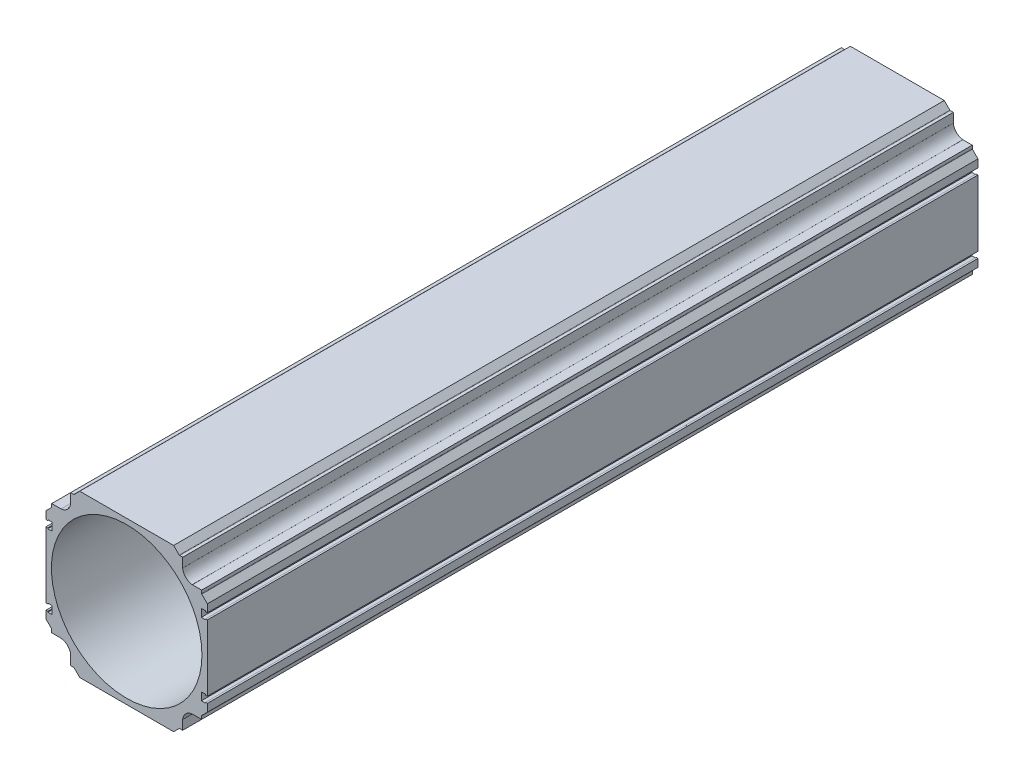
SolidWorks part; units mm, degrees
ref_plane "Front Plane" through (0, 0, 0) normal (0, 0, 1) x (1, 0, 0)
ref_plane "Top Plane" through (0, 0, 0) normal (0, 1, 0) x (1, 0, 0)
ref_plane "Right Plane" through (0, 0, 0) normal (1, 0, 0) x (0, 0, -1)
sketch "Sketch1" plane through (0, 0, 0) normal (0, 0, 1) x (1, 0, 0)
  line L0 (-68.7506, 0) -> (56.2494, 0) construction
  circle A0 centre (-6.2506, 0) radius 62.5
  spline S2 degree 3 poles (60.7494, -32.575) (60.2494, -32.575) (59.7494, -32.575) (59.2494, -32.575) knots 0 0 0 0 1 1 1 1
  spline S3 degree 3 poles (59.2494, -32.575) (59.2494, -32.8) (59.2494, -33.025) (59.2494, -33.25) knots 0 0 0 0 1 1 1 1
  spline S4 degree 3 poles (59.2494, -33.25) (58.0827, -33.25) (56.916, -33.25) (55.7494, -33.25) knots 0 0 0 0 1 1 1 1
  spline S5 degree 3 poles (55.7494, -33.25) (55.7494, -31.0833) (55.7494, -28.9167) (55.7494, -26.75) knots 0 0 0 0 1 1 1 1
  spline S6 degree 3 poles (55.7494, -26.75) (56.916, -26.75) (58.0827, -26.75) (59.2494, -26.75) knots 0 0 0 0 1 1 1 1
  spline S7 degree 3 poles (59.2494, -26.75) (59.2494, -26.975) (59.2494, -27.2) (59.2494, -27.425) knots 0 0 0 0 1 1 1 1
  spline S8 degree 3 poles (59.2494, -27.425) (59.7494, -27.425) (60.2494, -27.425) (60.7494, -27.425) knots 0 0 0 0 1 1 1 1
  spline S9 degree 3 poles (60.7494, -27.425) (60.7494, -9.1417) (60.7494, 9.1417) (60.7494, 27.425) knots 0 0 0 0 1 1 1 1
  spline S10 degree 3 poles (60.7494, 27.425) (60.2494, 27.425) (59.7494, 27.425) (59.2494, 27.425) knots 0 0 0 0 1 1 1 1
  spline S11 degree 3 poles (59.2494, 27.425) (59.2494, 27.2) (59.2494, 26.975) (59.2494, 26.75) knots 0 0 0 0 1 1 1 1
  spline S12 degree 3 poles (59.2494, 26.75) (58.0827, 26.75) (56.916, 26.75) (55.7494, 26.75) knots 0 0 0 0 1 1 1 1
  spline S13 degree 3 poles (55.7494, 26.75) (55.7494, 28.9167) (55.7494, 31.0833) (55.7494, 33.25) knots 0 0 0 0 1 1 1 1
  spline S14 degree 3 poles (55.7494, 33.25) (56.916, 33.25) (58.0827, 33.25) (59.2494, 33.25) knots 0 0 0 0 1 1 1 1
  spline S15 degree 3 poles (59.2494, 33.25) (59.2494, 33.025) (59.2494, 32.8) (59.2494, 32.575) knots 0 0 0 0 1 1 1 1
  spline S16 degree 3 poles (59.2494, 32.575) (59.7494, 32.575) (60.2494, 32.575) (60.7494, 32.575) knots 0 0 0 0 1 1 1 1
  spline S17 degree 3 poles (60.7494, 32.575) (60.7494, 34.7167) (60.7494, 36.8583) (60.7494, 39) knots 0 0 0 0 1 1 1 1
  spline S18 degree 3 poles (60.7494, 39) (59.2125, 40.5369) (57.6757, 42.0737) (56.1388, 43.6106) knots 0 0 0 0 1 1 1 1
  spline S19 degree 3 poles (56.1388, 43.6106) (56.0453, 43.7041) (55.9924, 43.8311) (55.9924, 43.9641) knots 0 0 0 0 1 1 1 1
  spline S20 degree 3 poles (55.9924, 43.9641) (55.9924, 44.8094) (55.9924, 45.6547) (55.9924, 46.5) knots 0 0 0 0 1 1 1 1
  spline S21 degree 3 poles (55.9924, 46.5) (53.4114, 46.5) (50.8304, 46.5) (48.2494, 46.5) knots 0 0 0 0 1 1 1 1
  spline S22 degree 3 poles (48.2494, 46.5) (48.2441, 46.5052) (48.2389, 46.5104) (48.2337, 46.5157) knots 0 0 0 0 1 1 1 1
  spline S23 degree 3 poles (48.2337, 46.5157) (44.1249, 46.7654) (40.5149, 50.3726) (40.265, 54.4843) knots 0 0 0 0 1 1 1 1
  spline S24 degree 3 poles (40.265, 54.4843) (40.2598, 54.4896) (40.2546, 54.4948) (40.2494, 54.5) knots 0 0 0 0 1 1 1 1
  spline S25 degree 3 poles (40.2494, 54.5) (40.2494, 57.081) (40.2494, 59.662) (40.2494, 62.243) knots 0 0 0 0 1 1 1 1
  spline S26 degree 3 poles (40.2494, 62.243) (39.4041, 62.243) (38.5588, 62.243) (37.7135, 62.243) knots 0 0 0 0 1 1 1 1
  spline S27 degree 3 poles (37.7135, 62.243) (37.5812, 62.243) (37.4539, 62.2954) (37.3599, 62.3894) knots 0 0 0 0 1 1 1 1
  spline S28 degree 3 poles (37.3599, 62.3894) (35.8231, 63.9263) (34.2862, 65.4631) (32.7494, 67) knots 0 0 0 0 1 1 1 1
  spline S29 degree 3 poles (32.7494, 67) (6.7494, 67) (-19.2506, 67) (-45.2506, 67) knots 0 0 0 0 1 1 1 1
  spline S30 degree 3 poles (-45.2506, 67) (-46.7875, 65.4631) (-48.3243, 63.9263) (-49.8612, 62.3894) knots 0 0 0 0 1 1 1 1
  spline S31 degree 3 poles (-49.8612, 62.3894) (-49.9547, 62.2959) (-50.0818, 62.243) (-50.2148, 62.243) knots 0 0 0 0 1 1 1 1
  spline S32 degree 3 poles (-50.2148, 62.243) (-51.0601, 62.243) (-51.9053, 62.243) (-52.7506, 62.243) knots 0 0 0 0 1 1 1 1
  spline S33 degree 3 poles (-52.7506, 62.243) (-52.7506, 59.662) (-52.7506, 57.081) (-52.7506, 54.5) knots 0 0 0 0 1 1 1 1
  spline S34 degree 3 poles (-52.7506, 54.5) (-52.7559, 54.4948) (-52.7611, 54.4896) (-52.7663, 54.4843) knots 0 0 0 0 1 1 1 1
  spline S35 degree 3 poles (-52.7663, 54.4843) (-53.016, 50.3755) (-56.6232, 46.7656) (-60.735, 46.5157) knots 0 0 0 0 1 1 1 1
  spline S36 degree 3 poles (-60.735, 46.5157) (-60.7402, 46.5104) (-60.7454, 46.5052) (-60.7506, 46.5) knots 0 0 0 0 1 1 1 1
  spline S37 degree 3 poles (-60.7506, 46.5) (-63.3316, 46.5) (-65.9126, 46.5) (-68.4936, 46.5) knots 0 0 0 0 1 1 1 1
  spline S38 degree 3 poles (-68.4936, 46.5) (-68.4936, 45.6547) (-68.4936, 44.8094) (-68.4936, 43.9641) knots 0 0 0 0 1 1 1 1
  spline S39 degree 3 poles (-68.4936, 43.9641) (-68.4936, 43.8319) (-68.5461, 43.7046) (-68.6401, 43.6106) knots 0 0 0 0 1 1 1 1
  spline S40 degree 3 poles (-68.6401, 43.6106) (-70.1769, 42.0737) (-71.7138, 40.5369) (-73.2506, 39) knots 0 0 0 0 1 1 1 1
  spline S41 degree 3 poles (-73.2506, 39) (-73.2506, 36.8583) (-73.2506, 34.7167) (-73.2506, 32.575) knots 0 0 0 0 1 1 1 1
  spline S42 degree 3 poles (-73.2506, 32.575) (-72.7506, 32.575) (-72.2506, 32.575) (-71.7506, 32.575) knots 0 0 0 0 1 1 1 1
  spline S43 degree 3 poles (-71.7506, 32.575) (-71.7506, 32.8) (-71.7506, 33.025) (-71.7506, 33.25) knots 0 0 0 0 1 1 1 1
  spline S44 degree 3 poles (-71.7506, 33.25) (-70.584, 33.25) (-69.4173, 33.25) (-68.2506, 33.25) knots 0 0 0 0 1 1 1 1
  spline S45 degree 3 poles (-68.2506, 33.25) (-68.2506, 31.0833) (-68.2506, 28.9167) (-68.2506, 26.75) knots 0 0 0 0 1 1 1 1
  spline S46 degree 3 poles (-68.2506, 26.75) (-69.4173, 26.75) (-70.584, 26.75) (-71.7506, 26.75) knots 0 0 0 0 1 1 1 1
  spline S47 degree 3 poles (-71.7506, 26.75) (-71.7506, 26.975) (-71.7506, 27.2) (-71.7506, 27.425) knots 0 0 0 0 1 1 1 1
  spline S48 degree 3 poles (-71.7506, 27.425) (-72.2506, 27.425) (-72.7506, 27.425) (-73.2506, 27.425) knots 0 0 0 0 1 1 1 1
  spline S49 degree 3 poles (-73.2506, 27.425) (-73.2506, 9.1417) (-73.2506, -9.1417) (-73.2506, -27.425) knots 0 0 0 0 1 1 1 1
  spline S50 degree 3 poles (-73.2506, -27.425) (-72.7506, -27.425) (-72.2506, -27.425) (-71.7506, -27.425) knots 0 0 0 0 1 1 1 1
  spline S51 degree 3 poles (-71.7506, -27.425) (-71.7506, -27.2) (-71.7506, -26.975) (-71.7506, -26.75) knots 0 0 0 0 1 1 1 1
  spline S52 degree 3 poles (-71.7506, -26.75) (-70.584, -26.75) (-69.4173, -26.75) (-68.2506, -26.75) knots 0 0 0 0 1 1 1 1
  spline S53 degree 3 poles (-68.2506, -26.75) (-68.2506, -28.9167) (-68.2506, -31.0833) (-68.2506, -33.25) knots 0 0 0 0 1 1 1 1
  spline S54 degree 3 poles (-68.2506, -33.25) (-69.4173, -33.25) (-70.584, -33.25) (-71.7506, -33.25) knots 0 0 0 0 1 1 1 1
  spline S55 degree 3 poles (-71.7506, -33.25) (-71.7506, -33.025) (-71.7506, -32.8) (-71.7506, -32.575) knots 0 0 0 0 1 1 1 1
  spline S56 degree 3 poles (-71.7506, -32.575) (-72.2506, -32.575) (-72.7506, -32.575) (-73.2506, -32.575) knots 0 0 0 0 1 1 1 1
  spline S57 degree 3 poles (-73.2506, -32.575) (-73.2506, -34.7167) (-73.2506, -36.8583) (-73.2506, -39) knots 0 0 0 0 1 1 1 1
  spline S58 degree 3 poles (-73.2506, -39) (-71.7138, -40.5369) (-70.1769, -42.0737) (-68.6401, -43.6106) knots 0 0 0 0 1 1 1 1
  spline S59 degree 3 poles (-68.6401, -43.6106) (-68.5466, -43.7041) (-68.4936, -43.8311) (-68.4936, -43.9641) knots 0 0 0 0 1 1 1 1
  spline S60 degree 3 poles (-68.4936, -43.9641) (-68.4936, -44.8094) (-68.4936, -45.6547) (-68.4936, -46.5) knots 0 0 0 0 1 1 1 1
  spline S61 degree 3 poles (-68.4936, -46.5) (-65.9126, -46.5) (-63.3316, -46.5) (-60.7506, -46.5) knots 0 0 0 0 1 1 1 1
  spline S62 degree 3 poles (-60.7506, -46.5) (-60.7454, -46.5052) (-60.7402, -46.5104) (-60.735, -46.5157) knots 0 0 0 0 1 1 1 1
  spline S63 degree 3 poles (-60.735, -46.5157) (-56.6262, -46.7654) (-53.0162, -50.3726) (-52.7663, -54.4843) knots 0 0 0 0 1 1 1 1
  spline S64 degree 3 poles (-52.7663, -54.4843) (-52.7611, -54.4896) (-52.7559, -54.4948) (-52.7506, -54.5) knots 0 0 0 0 1 1 1 1
  spline S65 degree 3 poles (-52.7506, -54.5) (-52.7506, -57.081) (-52.7506, -59.662) (-52.7506, -62.243) knots 0 0 0 0 1 1 1 1
  spline S66 degree 3 poles (-52.7506, -62.243) (-51.9053, -62.243) (-51.0601, -62.243) (-50.2148, -62.243) knots 0 0 0 0 1 1 1 1
  spline S67 degree 3 poles (-50.2148, -62.243) (-50.0825, -62.243) (-49.9552, -62.2954) (-49.8612, -62.3894) knots 0 0 0 0 1 1 1 1
  spline S68 degree 3 poles (-49.8612, -62.3894) (-48.3243, -63.9263) (-46.7875, -65.4631) (-45.2506, -67) knots 0 0 0 0 1 1 1 1
  spline S69 degree 3 poles (-45.2506, -67) (-19.2506, -67) (6.7494, -67) (32.7494, -67) knots 0 0 0 0 1 1 1 1
  spline S70 degree 3 poles (32.7494, -67) (34.2862, -65.4631) (35.8231, -63.9263) (37.3599, -62.3894) knots 0 0 0 0 1 1 1 1
  spline S71 degree 3 poles (37.3599, -62.3894) (37.4534, -62.2959) (37.5805, -62.243) (37.7135, -62.243) knots 0 0 0 0 1 1 1 1
  spline S72 degree 3 poles (37.7135, -62.243) (38.5588, -62.243) (39.4041, -62.243) (40.2494, -62.243) knots 0 0 0 0 1 1 1 1
  spline S73 degree 3 poles (40.2494, -62.243) (40.2494, -59.662) (40.2494, -57.081) (40.2494, -54.5) knots 0 0 0 0 1 1 1 1
  spline S74 degree 3 poles (40.2494, -54.5) (40.2546, -54.4948) (40.2598, -54.4896) (40.265, -54.4843) knots 0 0 0 0 1 1 1 1
  spline S75 degree 3 poles (40.265, -54.4843) (40.5147, -50.3755) (44.1219, -46.7656) (48.2337, -46.5157) knots 0 0 0 0 1 1 1 1
  spline S76 degree 3 poles (48.2337, -46.5157) (48.2389, -46.5104) (48.2441, -46.5052) (48.2494, -46.5) knots 0 0 0 0 1 1 1 1
  spline S77 degree 3 poles (48.2494, -46.5) (50.8304, -46.5) (53.4114, -46.5) (55.9924, -46.5) knots 0 0 0 0 1 1 1 1
  spline S78 degree 3 poles (55.9924, -46.5) (55.9924, -45.6547) (55.9924, -44.8094) (55.9924, -43.9641) knots 0 0 0 0 1 1 1 1
  spline S79 degree 3 poles (55.9924, -43.9641) (55.9924, -43.8319) (56.0448, -43.7046) (56.1388, -43.6106) knots 0 0 0 0 1 1 1 1
  spline S80 degree 3 poles (56.1388, -43.6106) (57.6757, -42.0737) (59.2125, -40.5369) (60.7494, -39) knots 0 0 0 0 1 1 1 1
  spline S81 degree 3 poles (60.7494, -39) (60.7494, -36.8583) (60.7494, -34.7167) (60.7494, -32.575) knots 0 0 0 0 1 1 1 1
extrude "Boss-Extrude1" add sketch "Sketch1" along normal blind 640
